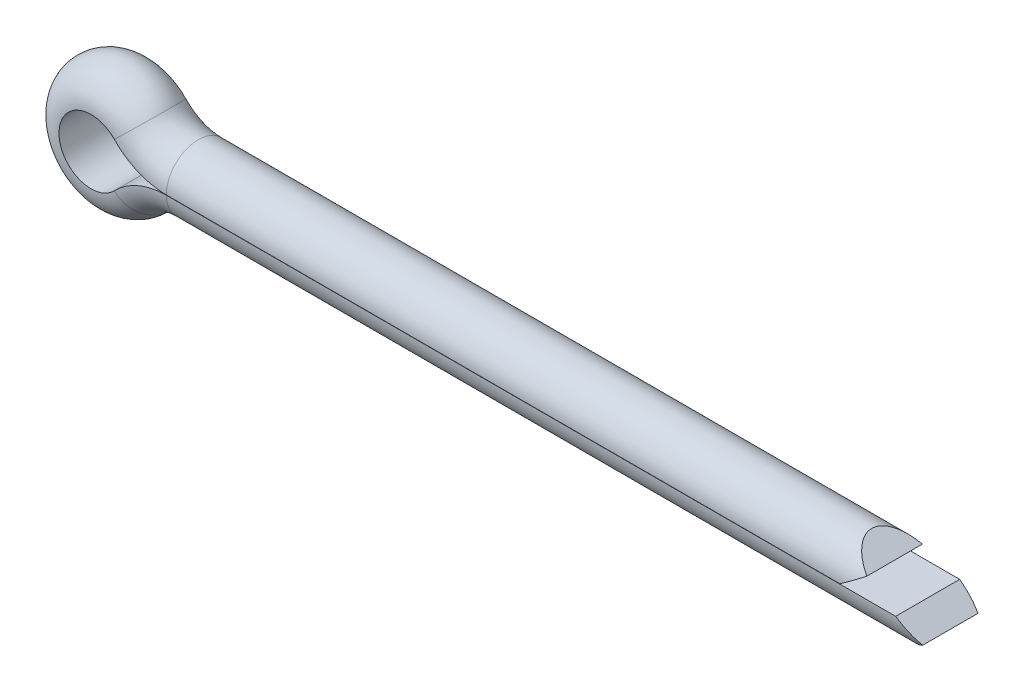
from build123d import *

# Parameters (mm, degrees)
CUT_EXTRUDE1_DEPTH      = 60.622226572
CUT_EXTRUDE1_DEPTH_BACK = 60.622226572


with BuildPart() as part:
    # Sweep2: sweep along a path in Dimension sketch
    with BuildLine(Plane.XY) as sweep2_path:
        Line((55.4, 2.3), (5.4, 2.3))
        ThreePointArc((5.4, 2.3), (4.267859381, 2.531061156), (3.316806967, 3.187285922))
        ThreePointArc((3.316806967, 3.187285922), (-4.6, 0), (3.316806967, -3.187285922))
        ThreePointArc((3.316806967, -3.187285922), (4.267859381, -2.531061156), (5.4, -2.3))
        Line((5.4, -2.3), (59.4, -2.3))
    # Sketch2 → Sweep2 (sweep)
    with BuildSketch(Plane(origin=(55.4, 2.3, 0), x_dir=(0, 0, 1), z_dir=(-1, 0, 0))):
        with BuildLine():
            Line((-2.299978261, -2.29), (2.299978261, -2.29))
            ThreePointArc((2.299978261, -2.29), (0, 0), (-2.299978261, -2.29))
        make_face()
    sweep(path=sweep2_path.line)

    # Sketch3 → Cut-Extrude1 (cut, two sides: drawn at the far end of the back side and taken through both)
    with BuildSketch(Plane.XY.offset(-CUT_EXTRUDE1_DEPTH_BACK)):
        Polygon((55.4, 1.145), (53.76113083, 2.3), (59.41, 2.3), (59.41, -2.3), (57.754128755, -2.3), (59.4, -1.155), (57.76113083, 0), (53.754128755, 0), align=None)
    extrude(amount=CUT_EXTRUDE1_DEPTH + CUT_EXTRUDE1_DEPTH_BACK, mode=Mode.SUBTRACT)


solid = part.part
